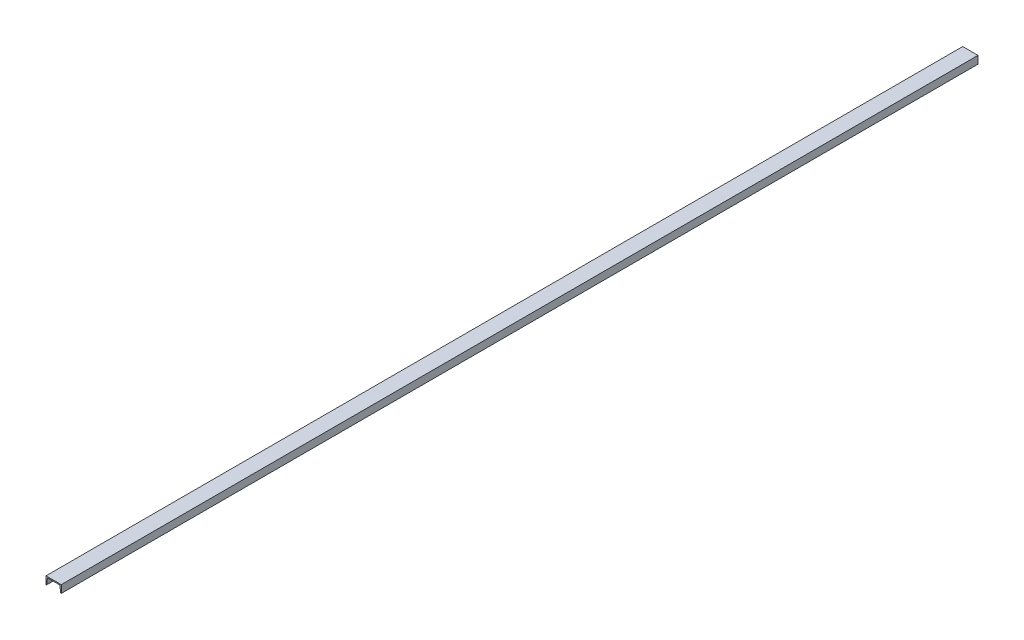
from build123d import *

# Parameters (mm, degrees)
BOSS_EXTRUDE1_DEPTH = 6000


with BuildPart() as part:
    # Sketch1 → Boss-Extrude1 (new body)
    with BuildSketch(Plane.XY):
        with BuildLine():
            Line((0, 0), (0, 50))
            Line((0, 50), (100, 50))
            Line((100, 50), (100, 0))
            Line((100, 0), (97.451472673, 0))
            ThreePointArc((97.451472673, 0), (96.119850629, 0.507759157), (95.464371872, 1.773217267))
            Line((95.464371872, 1.773217267), (91.247290138, 38.723854473))
            ThreePointArc((91.247290138, 38.723854473), (89.608593246, 41.887499748), (86.279538137, 43.156897641))
            Line((86.279538137, 43.156897641), (13.720461863, 43.156897641))
            ThreePointArc((13.720461863, 43.156897641), (10.391406754, 41.887499748), (8.752709862, 38.723854473))
            Line((8.752709862, 38.723854473), (4.535628128, 1.773217267))
            ThreePointArc((4.535628128, 1.773217267), (3.880149371, 0.507759157), (2.548527327, 0))
            Line((2.548527327, 0), (0, 0))
        make_face()
    extrude(amount=BOSS_EXTRUDE1_DEPTH)


solid = part.part
